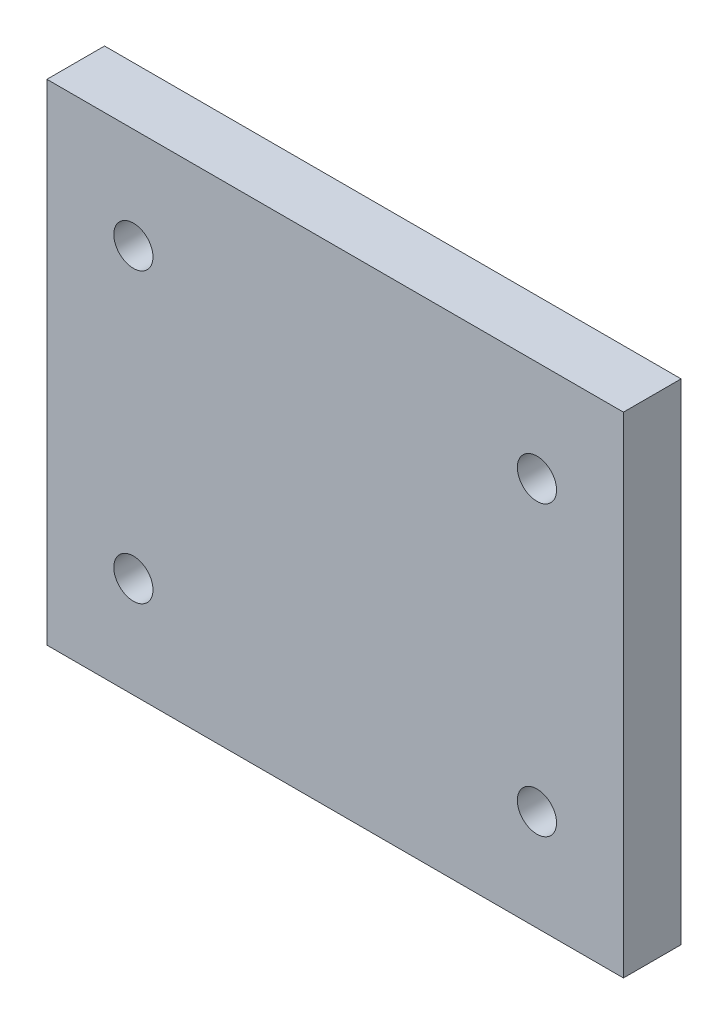
SolidWorks part; units mm, degrees
material "1023 碳钢板 (SS)"
ref_plane "Front Plane" through (0, 0, 0) normal (0, 0, 1) x (1, 0, 0)
ref_plane "Top Plane" through (0, 0, 0) normal (0, 1, 0) x (1, 0, 0)
ref_plane "Right Plane" through (0, 0, 0) normal (1, 0, 0) x (0, 0, -1)
sketch "Sketch1" plane through (0, 0, 0) normal (0, 0, 1) x (1, 0, 0)
  line L1 (50, 42.5) -> (-50, 42.5)
  line L2 (50, 42.5) -> (50, -42.5)
  line L3 (50, -42.5) -> (-50, -42.5)
  line L4 (-50, 42.5) -> (-50, -42.5)
  line L5 (50, 42.5) -> (-50, -42.5) construction
  line L6 (50, -42.5) -> (-50, 42.5) construction
  point P0 (0, 0)
  dimension "D1" = 100
  dimension "D2" = 85
extrude "Boss-Extrude1" add sketch "Sketch1" along normal blind 10
sketch "Sketch2" plane through (0, 0, 10) normal (0, 0, 1) x (1, 0, 0)
  circle A0 centre (-35, 25) radius 3
  circle A1 centre (35, 25) radius 3
  circle A2 centre (35, -25) radius 3
  circle A4 centre (-35, -25) radius 3
  dimension "D4" = 6
  dimension "D5" = 25
  dimension "D1" = 70
  dimension "D2" = 35
  dimension "D3" = 50
hole_wizard "M8 Tapped Hole1" positions "Sketch3" profile "Sketch4" tap size "M8" standard "ISO"
sketch "Sketch3" plane through (0, 0, 10) normal (0, 0, 1) x (1, 0, 0)
  point P0 (-35, 25)
  point P3 (35, 25)
  point P6 (35, -25)
  point P9 (-35, -25)
sketch "Sketch4" plane through (-35, 25, 10) normal (1, 0, 0) x (0, -1, 0)
  line L0 (0, 0) -> (0, 21.7929)
  line L1 (0, 21.7929) -> (3.4, 19.75)
  line L2 (3.4, 19.75) -> (3.4, 0)
  line L5 (3.4, 0) -> (0, 0)
  line L10 (0, 21.7929) -> (-3.4, 19.75) construction
  line L11 (0, -6.35) -> (0, 107.95) construction
  dimension "螺纹孔钻头直径" = 6.8
  dimension "螺纹孔钻头深度" = 19.75
  dimension "导头角度" = 118
cosmetic thread "Hole Thread Line 1"
cosmetic thread "Hole Thread Line 2"
cosmetic thread "Hole Thread Line 3"
cosmetic thread "Hole Thread Line 4"
